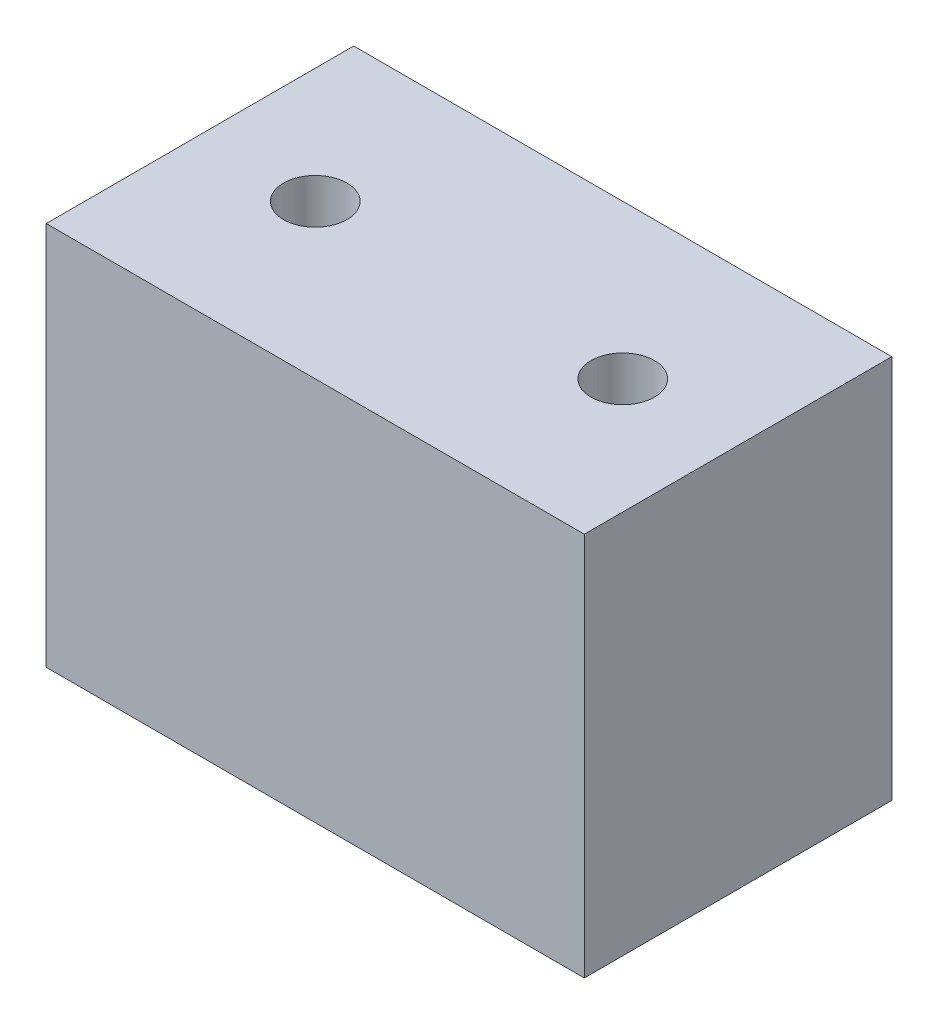
SolidWorks part; units mm, degrees
ref_plane "前视基准面" through (0, 0, 0) normal (0, 0, 1) x (1, 0, 0)
ref_plane "上视基准面" through (0, 0, 0) normal (0, 1, 0) x (1, 0, 0)
ref_plane "右视基准面" through (0, 0, 0) normal (1, 0, 0) x (0, 0, -1)
other "Configuration Table"
sketch "草图1" plane through (0, 0, 0) normal (0, 0, 1) x (1, 0, 0)
  line L0 (-14, -10) -> (14, -10)
  line L1 (14, -10) -> (14, 10)
  line L2 (14, 10) -> (-14, 10)
  line L3 (-14, 10) -> (-14, -10)
  point P0 (0, 0)
  dimension "D1" = 14
  dimension "D2" = 28
  dimension "D3" = 10
  dimension "D4" = 20
extrude "凸台-拉伸1" add sketch "草图1" against normal mid plane 16
sketch "草图2" plane through (0, 0, 0) normal (0, 1, 0) x (1, 0, 0)
  circle A0 centre (-8, 0) radius 1.65
  circle A1 centre (8, 0) radius 1.65
  point P0 (0, 0)
  dimension "D1" = 3.3
  dimension "D2" = 3.3
  dimension "D3" = 8
  dimension "D4" = 16
extrude "切除-拉伸1" cut sketch "草图2" against normal mid plane 26
